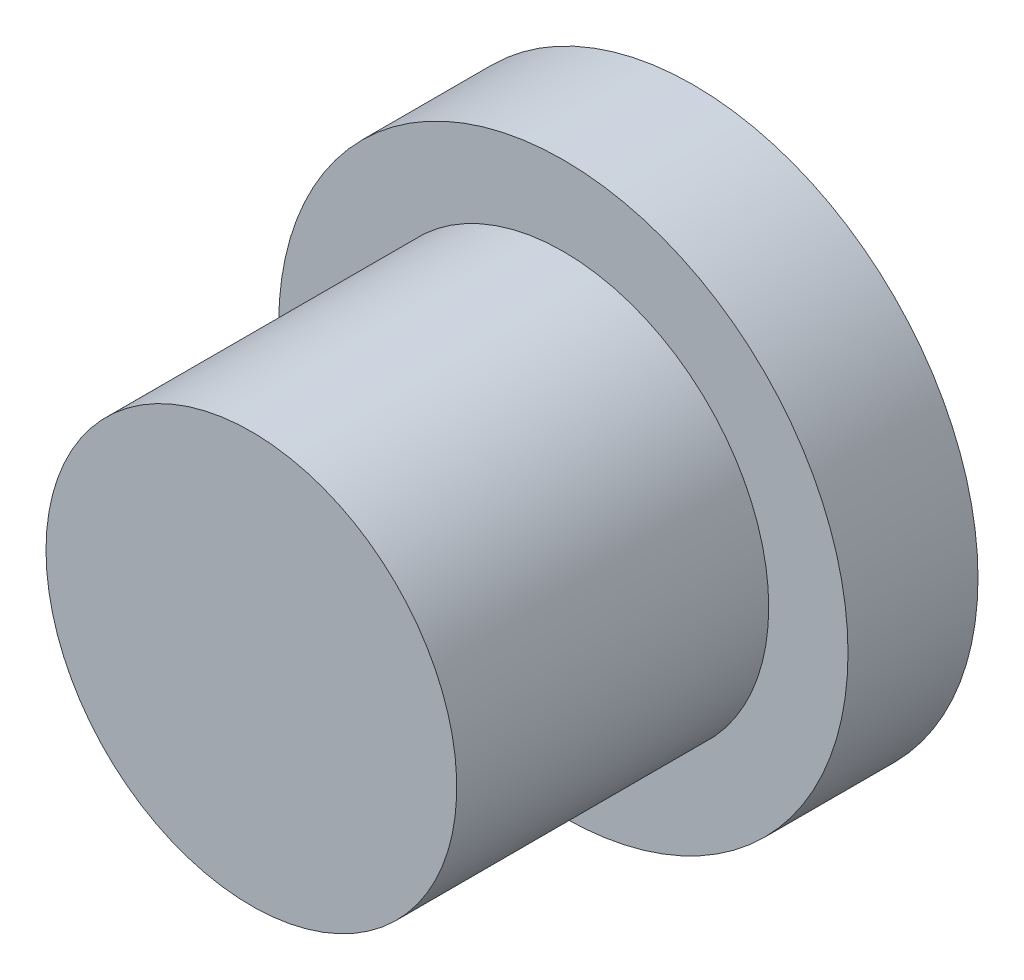
SolidWorks part; units mm, degrees
ref_plane "前视基准面" through (0, 0, 0) normal (0, 0, 1) x (1, 0, 0)
ref_plane "上视基准面" through (0, 0, 0) normal (0, 1, 0) x (1, 0, 0)
ref_plane "右视基准面" through (0, 0, 0) normal (1, 0, 0) x (0, 0, -1)
sketch "草图1" plane through (0, 0, 0) normal (0, 0, 1) x (1, 0, 0)
  circle A0 centre (0, 0) radius 10.95
  dimension "D1" = 21.9
extrude "凸台-拉伸1" add sketch "草图1" along normal blind 5
sketch "草图2" plane through (0, 0, 0) normal (0, 0, -1) x (-1, 0, 0)
  circle A0 centre (0, 0) radius 7.9
  dimension "D1" = 15.8
extrude "凸台-拉伸2" add sketch "草图2" against normal blind 17
sketch "草图3" plane through (0, 0, 0) normal (0, 0, -1) x (-1, 0, 0)
  line L1 (0, 4.7343) -> (-4.1, 2.3671)
  line L2 (-4.1, 2.3671) -> (-4.1, -2.3671)
  line L3 (-4.1, -2.3671) -> (0, -4.7343)
  line L4 (0, -4.7343) -> (4.1, -2.3671)
  line L5 (4.1, -2.3671) -> (4.1, 2.3671)
  line L6 (4.1, 2.3671) -> (0, 4.7343)
  circle A0 centre (0, 0) radius 4.1 construction
  point P1 (-4.1, 0)
  dimension "D1" = 8.2
extrude "切除-拉伸1" cut sketch "草图3" against normal blind 5
